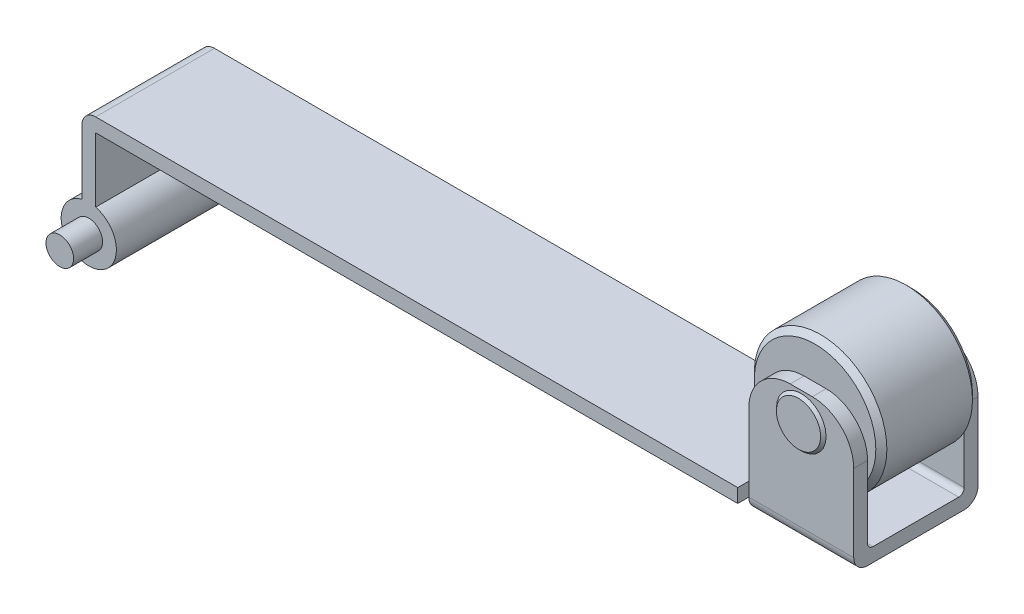
from build123d import *

# Parameters (mm, degrees)
SKETCH_1_R          = 0.5
EXTRUDE_1_DEPTH     = 2.15
SKETCH_2_R          = 0.5
EXTRUDE_2_DEPTH     = 3.2
EXTRUDE_3_DEPTH     = 3.8
FILLET_2_R          = 0.2
SKETCH_4_W          = 0.5
SKETCH_4_H          = 0.65
CUT_EXTRUDE_1_DEPTH = 29.392252464
FILLET_3_R          = 0.5
SKETCH_5_R          = 1
EXTRUDE_4_DEPTH     = 2.35
CHAMFER_1_SIZE      = 0.2
SKETCH_6_R          = 2.4
EXTRUDE_5_DEPTH     = 1.75
CHAMFER_2_SIZE      = 0.2
FILLET_4_R          = 1.5


with BuildPart() as part:
    # 草图1 → 凸台-拉伸1 (new, symmetric)
    with BuildSketch(Plane.XY):
        with BuildLine():
            Line((-0.25, 3.3), (-0.25, 0.968245837))
            ThreePointArc((-0.25, 0.968245837), (0, -1), (0.25, 0.968245837))
            Line((0.25, 0.968245837), (0.25, 3.3))
            Line((0.25, 3.3), (27.8, 3.3))
            Line((27.8, 3.3), (27.8, 3.8))
            Line((27.8, 3.8), (0.25, 3.8))
            ThreePointArc((0.25, 3.8), (-0.103553391, 3.653553391), (-0.25, 3.3))
        make_face()
        Circle(SKETCH_1_R, mode=Mode.SUBTRACT)
    extrude(amount=EXTRUDE_1_DEPTH, both=True)

    # 草图2 → 凸台-拉伸2 (add, symmetric)
    with BuildSketch(Plane.XY):
        Circle(SKETCH_2_R)
    extrude(amount=EXTRUDE_2_DEPTH, both=True)

    # 草图3 → 凸台-拉伸3 (add)
    with BuildSketch(Plane(origin=(27.8, 0, 0), x_dir=(0, 0, -1), z_dir=(1, 0, 0))):
        Polygon((-2.15, 3.8), (-1.75, 3.8), (-1.75, 8.1), (-2.25, 8.1), (-2.25, 3.3), (-2.15, 3.3), align=None)
        Polygon((2.15, 3.3), (2.25, 3.3), (2.25, 8.1), (1.75, 8.1), (1.75, 3.8), (2.15, 3.8), align=None)
    extrude(amount=-EXTRUDE_3_DEPTH)

    # 圆角2
    fillet_2_edges = [part.edges().sort_by_distance(p)[0] for p in [
        (25.9, 3.8, -1.75),
        (25.9, 3.8, 1.75),
    ]]
    fillet(fillet_2_edges, radius=FILLET_2_R)

    # 草图4 → 切除-拉伸1 (cut, through all)
    with BuildSketch(Plane(origin=(0, 3.8, 0), x_dir=(1, 0, 0), z_dir=(0, 1, 0))):
        with Locations((23.75, -1.925)):
            Rectangle(SKETCH_4_W, SKETCH_4_H)
        with Locations((23.75, 1.925)):
            Rectangle(SKETCH_4_W, SKETCH_4_H)
    extrude(amount=-CUT_EXTRUDE_1_DEPTH, mode=Mode.SUBTRACT)

    # 圆角3
    fillet_3_edges = [part.edges().sort_by_distance(p)[0] for p in [
        (25.9, 3.3, -2.25),
        (25.9, 3.3, 2.25),
    ]]
    fillet(fillet_3_edges, radius=FILLET_3_R)

    # 圆角4
    fillet_4_edges = [part.edges().sort_by_distance(p)[0] for p in [
        (24, 8.1, -2),
        (27.8, 8.1, -2),
        (24, 8.1, 2),
        (27.8, 8.1, 2),
    ]]
    fillet(fillet_4_edges, radius=FILLET_4_R)


with BuildPart() as body_2:
    # 草图5 → 凸台-拉伸4 (new, symmetric)
    with BuildSketch(Plane.XY):
        with Locations(Location((25.9, 7.1, 0), (0, 0, 180))):
            Circle(SKETCH_5_R)
    extrude(amount=EXTRUDE_4_DEPTH, both=True)

    # 倒角1
    chamfer_1_edges = [body_2.edges().sort_by_distance(p)[0] for p in [
        (26.9, 7.1, -2.35),
        (26.9, 7.1, 2.35),
    ]]
    chamfer(chamfer_1_edges, length=CHAMFER_1_SIZE)


with BuildPart() as body_3:
    # 草图6 → 凸台-拉伸5 (new, symmetric)
    with BuildSketch(Plane.XY):
        with Locations((25.9, 7.1)):
            Circle(SKETCH_6_R)
    extrude(amount=EXTRUDE_5_DEPTH, both=True)

    # 倒角2
    chamfer_2_edges = [body_3.edges().sort_by_distance(p)[0] for p in [
        (23.5, 7.1, -1.75),
        (23.5, 7.1, 1.75),
    ]]
    chamfer(chamfer_2_edges, length=CHAMFER_2_SIZE)


solid = Compound([part.part, body_2.part, body_3.part])
